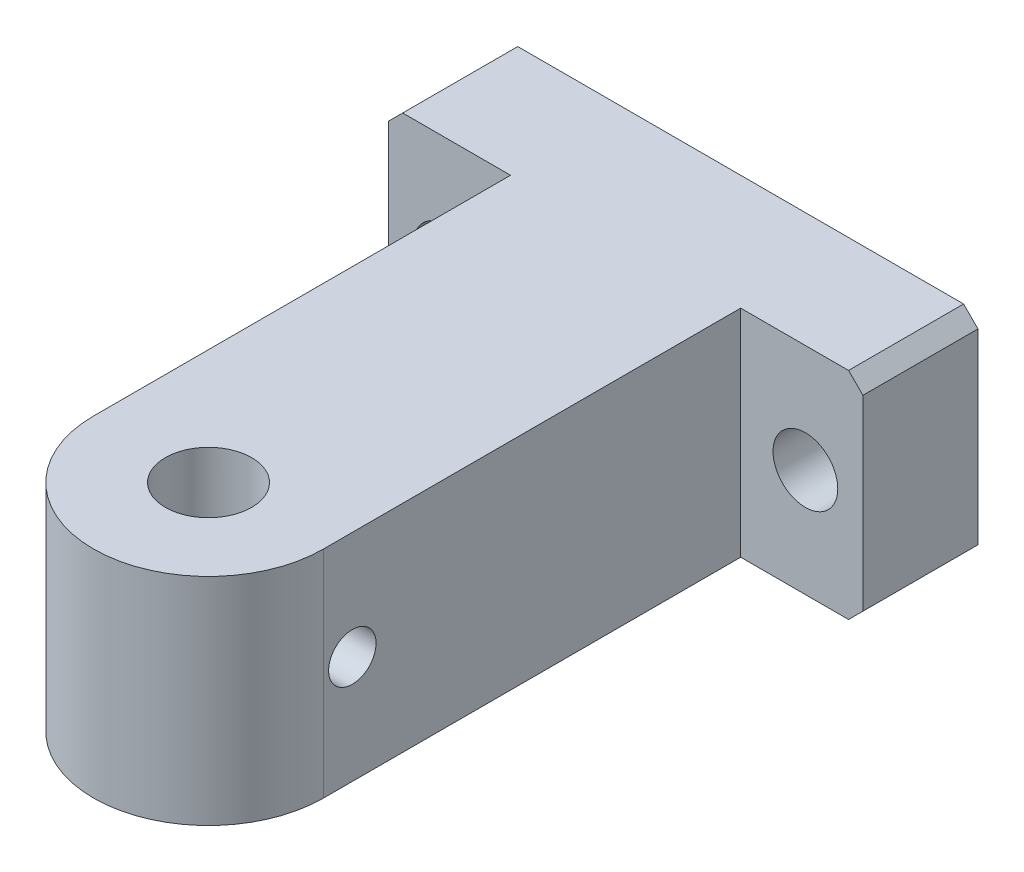
from build123d import *

# Parameters (mm, degrees)
SKETCH_1_R          = 3
EXTRUDE_1_DEPTH     = 7.5
HOLE_WIZARD_M4_1_D  = 3.3
SKETCH_5_R          = 2.25
CUT_EXTRUDE_1_DEPTH = 10
CHAMFER_1_SIZE      = 1


with BuildPart() as part:
    # 草图1 → 凸台-拉伸1 (new, symmetric)
    with BuildSketch(Plane(origin=(0, 0, 0), x_dir=(1, 0, 0), z_dir=(0, 1, 0))):
        with BuildLine():
            Line((-8, 0), (-8, 29))
            Line((-8, 29), (-16.5, 29))
            Line((-16.5, 29), (-16.5, 37))
            Line((-16.5, 37), (16.5, 37))
            Line((16.5, 37), (16.5, 29))
            Line((16.5, 29), (8, 29))
            Line((8, 29), (8, 0))
            ThreePointArc((8, 0), (0, -8), (-8, 0))
        make_face()
        with Locations(Location((0, 0, 0), (0, 0, 270))):
            Circle(SKETCH_1_R, mode=Mode.SUBTRACT)
    extrude(amount=EXTRUDE_1_DEPTH, both=True)

    # M4 螺纹孔1 (through all)
    with Locations(Plane(origin=(8, 0, 0), x_dir=(0, 0, -1), z_dir=(1, 0, 0))):
        with Locations((2, 0)):
            Hole(HOLE_WIZARD_M4_1_D / 2)

    # 草图5 → 切除-拉伸1 (cut)
    with BuildSketch(Plane.XY.offset(-29)):
        with Locations((-12.5, 0)):
            Circle(SKETCH_5_R)
        with Locations((12.5, 0)):
            Circle(SKETCH_5_R)
    extrude(amount=-CUT_EXTRUDE_1_DEPTH, mode=Mode.SUBTRACT)

    # 倒角1
    chamfer_1_edges = [part.edges().sort_by_distance(p)[0] for p in [
        (16.5, 7.5, -33),
        (-16.5, 7.5, -33),
        (-16.5, -7.5, -33),
        (16.5, -7.5, -33),
    ]]
    chamfer(chamfer_1_edges, length=CHAMFER_1_SIZE)


solid = part.part
